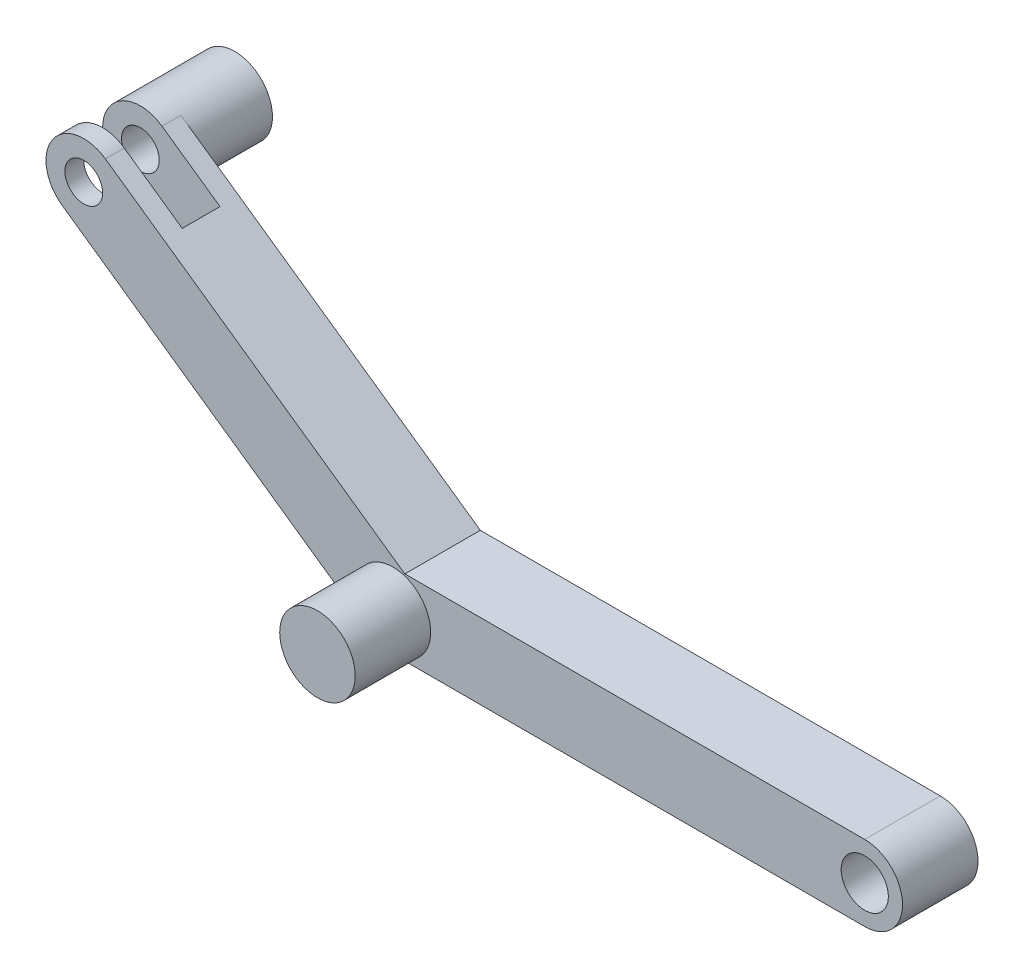
from build123d import *

# Parameters (mm, degrees)
BOSS_EXTRUDE1_DEPTH = 16
SKETCH2_R           = 5
CUT_EXTRUDE1_DEPTH  = 16
SKETCH3_R           = 8
BOSS_EXTRUDE2_DEPTH = 32
BOSS_EXTRUDE3_START = -32
SKETCH4_R           = 8
BOSS_EXTRUDE3_DEPTH = 32
SKETCH5_W           = 30
SKETCH5_H           = 8
CUT_EXTRUDE2_DEPTH  = 38
SKETCH6_R           = 4
CUT_EXTRUDE3_DEPTH  = 38


with BuildPart() as part:
    # Sketch1 → Boss-Extrude1 (new body)
    with BuildSketch(Plane.XY):
        with BuildLine():
            Line((0, 8), (-97.477609689, 8))
            Line((-97.477609689, 8), (-160.943552052, 52.439331262))
            ThreePointArc((-160.943552052, 52.439331262), (-172.085379897, 50.474726399), (-170.120775034, 39.332898554))
            Line((-170.120775034, 39.332898554), (-102.522390311, -8))
            Line((-102.522390311, -8), (0, -8))
            ThreePointArc((0, -8), (8, 0), (0, 8))
        make_face()
    extrude(amount=BOSS_EXTRUDE1_DEPTH)

    # Sketch2 → Cut-Extrude1 (cut)
    with BuildSketch(Plane.XY.offset(16)):
        Circle(SKETCH2_R)
    extrude(amount=-CUT_EXTRUDE1_DEPTH, mode=Mode.SUBTRACT)

    # Sketch3 → Boss-Extrude2 (add)
    with BuildSketch(Plane(origin=(0, 0, 0), x_dir=(-1, 0, 0), z_dir=(0, 0, -1))):
        with Locations((100, 0)):
            Circle(SKETCH3_R)
    extrude(amount=-BOSS_EXTRUDE2_DEPTH)

    # Sketch4 → Boss-Extrude3 (add)
    with BuildSketch(Plane.XY.offset(16).offset(BOSS_EXTRUDE3_START)):
        with Locations(Location((-165.532163543, 45.886114908, 0), (0, 0, 235))):
            Circle(SKETCH4_R)
    extrude(amount=BOSS_EXTRUDE3_DEPTH)

    # Sketch5 → Cut-Extrude2 (cut)
    with BuildSketch(Plane(origin=(-37.487604325, -53.537847394, 0), x_dir=(0.819152044288991, -0.5735764363510472, 0), z_dir=(-0.5735764363510472, -0.819152044288991, 0))):
        with Locations((-161.915204429, 8)):
            Rectangle(SKETCH5_W, SKETCH5_H)
    extrude(amount=-CUT_EXTRUDE2_DEPTH, mode=Mode.SUBTRACT)

    # Sketch6 → Cut-Extrude3 (cut)
    with BuildSketch(Plane.XY.offset(16)):
        with Locations((-165.532163543, 45.886114908)):
            Circle(SKETCH6_R)
    extrude(amount=-CUT_EXTRUDE3_DEPTH, mode=Mode.SUBTRACT)


solid = part.part
